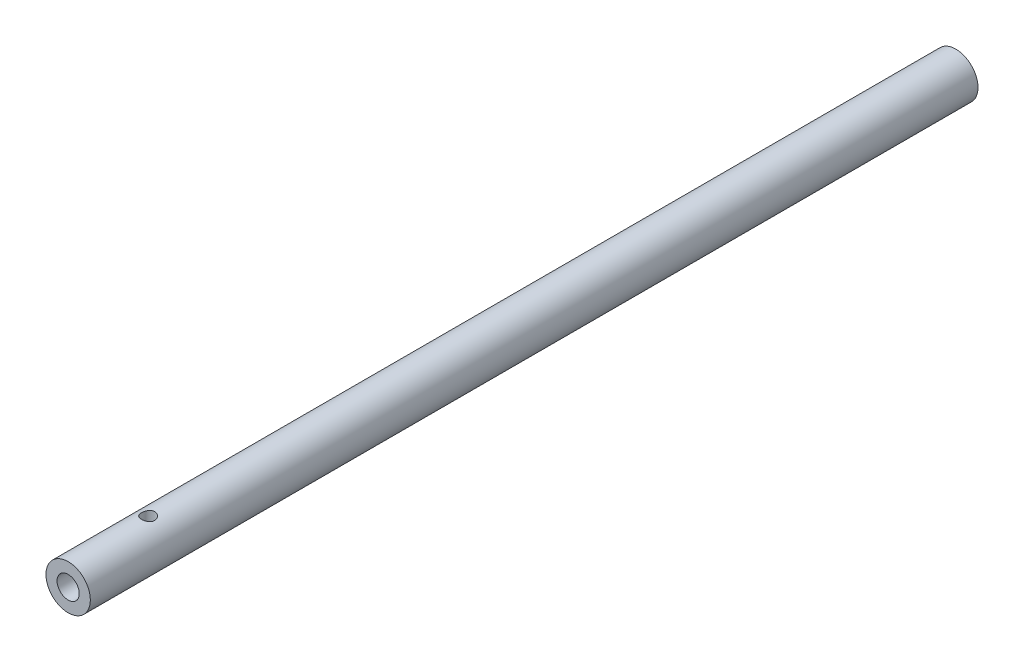
from build123d import *

# Parameters (mm, degrees)
SKETCH2_R               = 2.5
SKETCH2_R_2             = 1.25
BOSS_EXTRUDE1_DEPTH     = 100
CUT_EXTRUDE1_REACH      = 102.156
CUT_EXTRUDE1_END_RADIUS = 1.25
SKETCH3_R               = 0.75


with BuildPart() as part:
    # Sketch2 → Boss-Extrude1 (new body)
    with BuildSketch(Plane.XY):
        Circle(SKETCH2_R)
        Circle(SKETCH2_R_2, mode=Mode.SUBTRACT)
    extrude(amount=BOSS_EXTRUDE1_DEPTH)

    # Cut-Extrude1: up to this cylinder (the profile starts outside it)
    cut_extrude1_end = Plane(origin=(0, 0, 91), z_dir=(0, 0, -1)) * Cylinder(CUT_EXTRUDE1_END_RADIUS, 207.812, mode=Mode.PRIVATE)
    # Sketch3 → Cut-Extrude1 (cut, up to the surface)
    with BuildSketch(Plane(origin=(0, 2.5, 0), x_dir=(1, 0, 0), z_dir=(0, 1, 0)), mode=Mode.PRIVATE) as cut_extrude1_sk1:
        with Locations(Location((0, -91, 0), (0, 0, 270))):
            Circle(SKETCH3_R)
    cut_extrude1_tool1 = extrude(cut_extrude1_sk1.sketch, amount=-CUT_EXTRUDE1_REACH, mode=Mode.PRIVATE) - cut_extrude1_end
    add(cut_extrude1_tool1.solids().sort_by_distance((0, 2.5, 91))[0], mode=Mode.SUBTRACT)


solid = part.part
